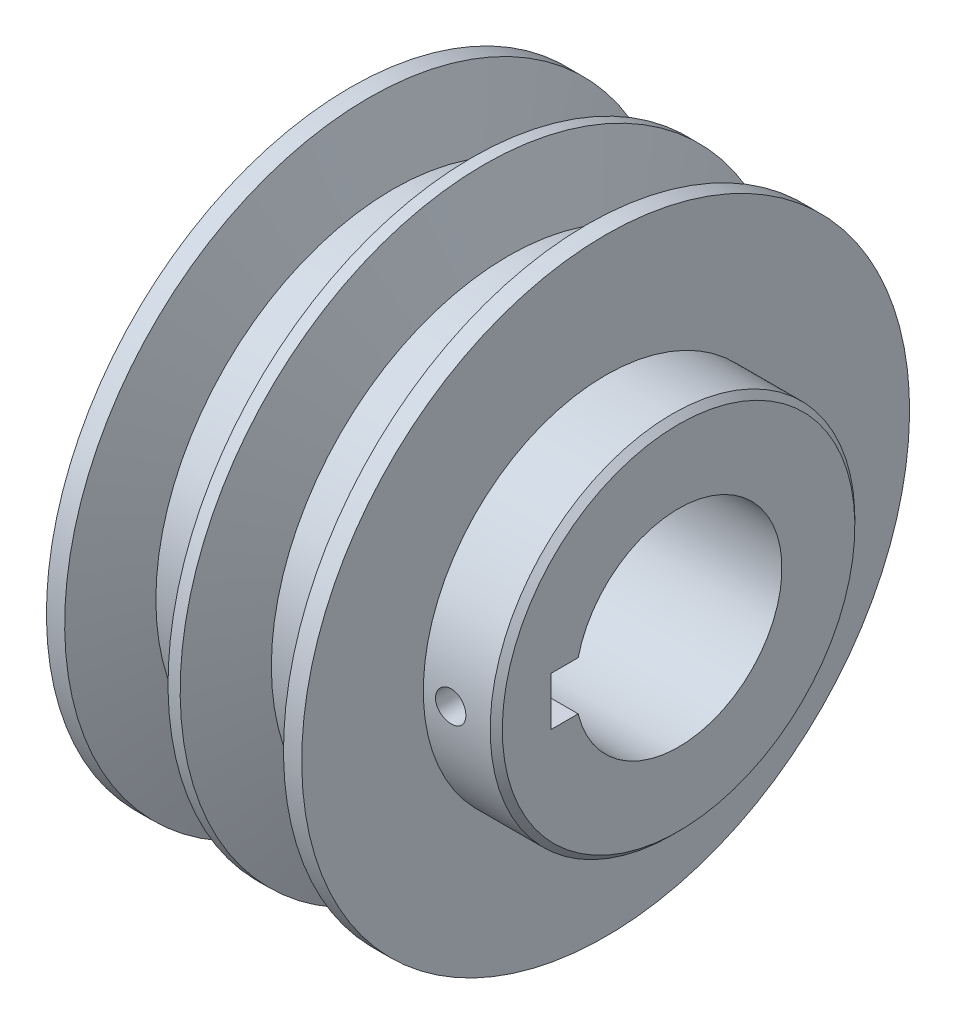
from build123d import *

# Parameters (mm, degrees)
SKETCH2_R          = 17
CUT_EXTRUDE1_DEPTH = 70
CHAMFER1_SIZE      = 1
SKETCH7_W          = 8
SKETCH7_H          = 8
CUT_EXTRUDE2_DEPTH = 70


with BuildPart() as part:
    # Sketch1 → Revolve1 (revolve)
    with BuildSketch(Plane.XY):
        Polygon((0, 0), (0, 50), (3, 50), (7.003672577, 39), (15.996327423, 39), (20, 50), (22, 50), (26.003672577, 39), (34.996327423, 39), (39, 50), (42, 50), (42, 30), (54, 30), (54, 0), align=None)
    revolve(axis=Axis((54, 0, 0), (-1, 0, 0)))

    # Sketch2 → Cut-Extrude1 (cut)
    with BuildSketch(Plane(origin=(54, 0, 0), x_dir=(0, 0, -1), z_dir=(1, 0, 0))):
        with Locations(Location((0, 0, 0), (0, 0, 90))):
            Circle(SKETCH2_R)
    extrude(amount=-CUT_EXTRUDE1_DEPTH, mode=Mode.SUBTRACT)

    # Sketch5 → M6 Tapped Hole1 (revolve, cut)
    with BuildSketch(Plane.YZ.offset(46.5)):
        Polygon((0, 0), (0, 51.502151548), (2.5, 50), (2.5, 0), align=None)
    revolve(axis=Axis((46.5, 0, -6.35), (0, 0, 1)), mode=Mode.SUBTRACT)

    # Chamfer1
    chamfer1_edges = [part.edges().sort_by_distance(p)[0] for p in [
        (54, -30, 0),
    ]]
    chamfer(chamfer1_edges, length=CHAMFER1_SIZE)

    # Sketch7 → Cut-Extrude2 (cut)
    with BuildSketch(Plane(origin=(54, 0, 0), x_dir=(0, 0, -1), z_dir=(1, 0, 0))):
        with Locations((-17, 0)):
            Rectangle(SKETCH7_W, SKETCH7_H)
    extrude(amount=-CUT_EXTRUDE2_DEPTH, mode=Mode.SUBTRACT)


solid = part.part
